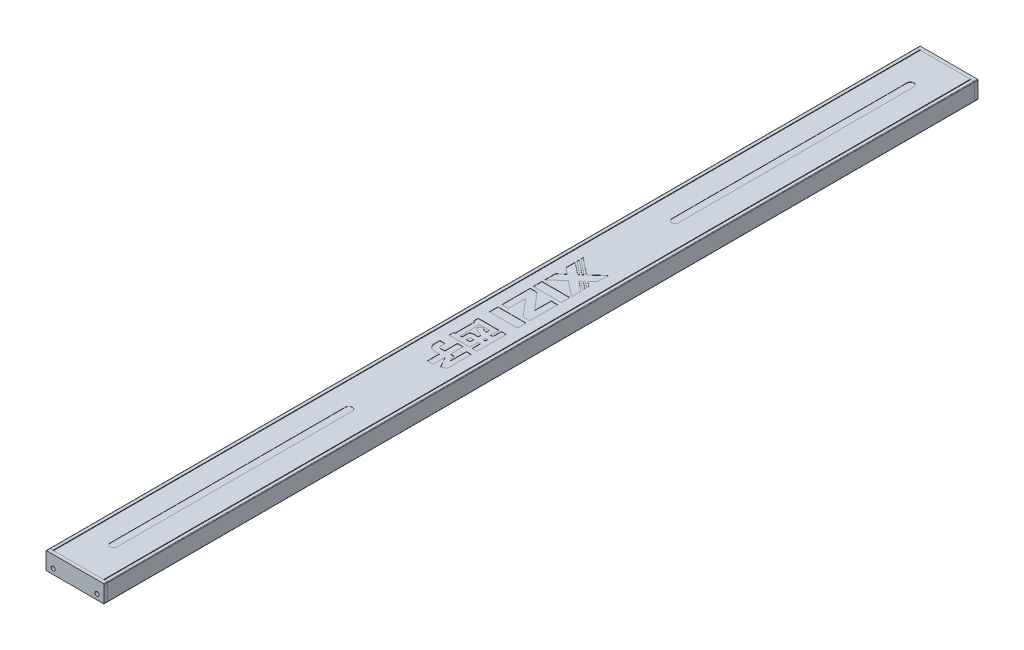
from build123d import *

# Parameters (mm, degrees)
EXTRUDE_1_DEPTH     = 372
SKETCH_3_W          = 43
SKETCH_3_H          = 744
EXTRUDE_4_DEPTH     = 6
SKETCH_7_W          = 50
SKETCH_7_H          = 15
SKETCH_7_R          = 1.75
EXTRUDE_3_DEPTH     = 3
FILLET_2_R          = 0.5
FILLET_3_R          = 0.5
SKETCH_13_W         = 24
SKETCH_13_H         = 7.373249396
SKETCH_13_H_2       = 7.373336991
SKETCH_13_W_2       = 1.89342737
SKETCH_13_H_3       = 1.872448876
CUT_EXTRUDE_1_DEPTH = 0.2


with BuildPart() as part:
    # 草图1 → 凸台-拉伸1 (new, symmetric)
    with BuildSketch(Plane.XY):
        with BuildLine():
            Line((22, 15), (24.5, 15))
            ThreePointArc((24.5, 15), (24.853553391, 14.853553391), (25, 14.5))
            Line((25, 14.5), (25, 0.5))
            ThreePointArc((25, 0.5), (24.853553391, 0.146446609), (24.5, 0))
            Line((24.5, 0), (20.866025404, 0))
            ThreePointArc((20.866025404, 0), (20, 0.5), (19.133974596, 0))
            Line((19.133974596, 0), (17.866025404, 0))
            ThreePointArc((17.866025404, 0), (17, 0.5), (16.133974596, 0))
            Line((16.133974596, 0), (14.866025404, 0))
            ThreePointArc((14.866025404, 0), (14, 0.5), (13.133974596, 0))
            Line((13.133974596, 0), (11.866025404, 0))
            ThreePointArc((11.866025404, 0), (11, 0.5), (10.133974596, 0))
            Line((10.133974596, 0), (-10.133974596, 0))
            ThreePointArc((-10.133974596, 0), (-11, 0.5), (-11.866025404, 0))
            Line((-11.866025404, 0), (-13.133974596, 0))
            ThreePointArc((-13.133974596, 0), (-14, 0.5), (-14.866025404, 0))
            Line((-14.866025404, 0), (-16.133974596, 0))
            ThreePointArc((-16.133974596, 0), (-17, 0.5), (-17.866025404, 0))
            Line((-17.866025404, 0), (-19.133974596, 0))
            ThreePointArc((-19.133974596, 0), (-20, 0.5), (-20.866025404, 0))
            Line((-20.866025404, 0), (-24.5, 0))
            ThreePointArc((-24.5, 0), (-24.853553391, 0.146446609), (-25, 0.5))
            Line((-25, 0.5), (-25, 14.5))
            ThreePointArc((-25, 14.5), (-24.853553391, 14.853553391), (-24.5, 15))
            Line((-24.5, 15), (-22, 15))
            Line((-22, 15), (-22, 9))
            Line((-22, 9), (-13, 9))
            Line((-13, 9), (-13, 8))
            Line((-13, 8), (-14.8, 8))
            ThreePointArc((-14.8, 8), (-14.941421356, 7.941421356), (-15, 7.8))
            Line((-15, 7.8), (-15, 2.7))
            ThreePointArc((-15, 2.7), (-14.941421356, 2.558578644), (-14.8, 2.5))
            Line((-14.8, 2.5), (14.8, 2.5))
            ThreePointArc((14.8, 2.5), (14.941421356, 2.558578644), (15, 2.7))
            Line((15, 2.7), (15, 7.8))
            ThreePointArc((15, 7.8), (14.941421356, 7.941421356), (14.8, 8))
            Line((14.8, 8), (13, 8))
            Line((13, 8), (13, 9))
            Line((13, 9), (22, 9))
            Line((22, 9), (22, 15))
        make_face()
        with BuildLine():
            Line((-21.011700936, 7), (-23, 7))
            Line((-23, 7), (-23, 2))
            Line((-23, 2), (-21.011700936, 2))
            Line((-21.011700936, 2), (-21.011700936, 2.838299064))
            ThreePointArc((-21.011700936, 2.838299064), (-20.672176824, 3.346432807), (-20.072792206, 3.227207794))
            ThreePointArc((-20.072792206, 3.227207794), (-17, 4.5), (-20.072792206, 5.772792206))
            ThreePointArc((-20.072792206, 5.772792206), (-20.672176824, 5.653567193), (-21.011700936, 6.161700936))
            Line((-21.011700936, 6.161700936), (-21.011700936, 7))
        make_face(mode=Mode.SUBTRACT)
        with BuildLine():
            Line((21.011700936, 2.838299064), (21.011700936, 2))
            Line((21.011700936, 2), (23, 2))
            Line((23, 2), (23, 7))
            Line((23, 7), (21.011700936, 7))
            Line((21.011700936, 7), (21.011700936, 6.161700936))
            ThreePointArc((21.011700936, 6.161700936), (20.672176824, 5.653567193), (20.072792206, 5.772792206))
            ThreePointArc((20.072792206, 5.772792206), (17, 4.5), (20.072792206, 3.227207794))
            ThreePointArc((20.072792206, 3.227207794), (20.672176824, 3.346432807), (21.011700936, 2.838299064))
        make_face(mode=Mode.SUBTRACT)
    extrude(amount=EXTRUDE_1_DEPTH, both=True)

    # 草图3 → 凸台-拉伸4 (add)
    with BuildSketch(Plane(origin=(0, 9, 363), x_dir=(1, 0, 0), z_dir=(0, -1, 0))):
        with Locations((0, -363)):
            Rectangle(SKETCH_3_W, SKETCH_3_H)
    extrude(amount=-EXTRUDE_4_DEPTH)

    # 草图13 → 切除-拉伸1 (cut)
    # profile 1 of 8: a face of its own
    with BuildSketch(Plane(origin=(0, 15, 0), x_dir=(1, 0, 0), z_dir=(0, 1, 0))):
        with BuildLine():
            Line((2.974241772, -342), (2.974241772, -140))
            ThreePointArc((2.974241772, -140), (0, -137.025758228), (-2.974241772, -140))
            Line((-2.974241772, -140), (-2.974241772, -342))
            ThreePointArc((-2.974241772, -342), (0, -344.974241772), (2.974241772, -342))
        make_face()
    # profile 2 of 8: a face of its own
    with BuildSketch(Plane(origin=(0, 15, 0), x_dir=(1, 0, 0), z_dir=(0, 1, 0))):
        with BuildLine():
            Line((-2.974241772, 140), (-2.974241772, 342))
            ThreePointArc((-2.974241772, 342), (0, 344.974241772), (2.974241772, 342))
            Line((2.974241772, 342), (2.974241772, 140))
            ThreePointArc((2.974241772, 140), (0, 137.025758228), (-2.974241772, 140))
        make_face()
    # profile 3 of 8: a face of its own
    with BuildSketch(Plane(origin=(0, 15, 0), x_dir=(1, 0, 0), z_dir=(0, 1, 0))):
        Polygon((4.456261904, 54.720624259), (12, 48.692451578), (12, 50.577345914), (5.57614696, 55.708810517), (6.471044745, 56.504083804), (12, 52.088692179), (12, 53.973586515), (7.592433512, 57.493890566), (12, 61.392166226), (12, 70.550396944), (2.156182764, 61.840932727), (-12, 73.159495911), (-12, 71.271287619), (1.035290368, 60.84821705), (0.138772079, 60.056257767), (-12, 69.759430422), (-12, 67.87021479), (-0.977988762, 59.063034807), (-1.931998445, 58.223526141), (-12, 66.268295531), (-12, 58.243322568), (-6.697535727, 54.009485788), (-12, 49.317425953), (-12, 40.158308155), (-1.256657054, 49.660330439), (12, 39.065460697), (12, 47.089013968), (3.504266901, 53.877684796), align=None)
    # profile 4 of 8: a face of its own
    with BuildSketch(Plane(origin=(0, 15, 0), x_dir=(1, 0, 0), z_dir=(0, 1, 0))):
        Polygon((-7.091113811, 27.560714457), (-12, 27.560714457), (-12, 3.255607132), (-6.354237064, 3.255607132), (-6.354237064, 18.06583115), (5.641186107, 3.943620573), (5.720368151, 3.880373274), (5.799825971, 3.817856759), (5.879835345, 3.756801814), (5.960672049, 3.697939223), (6.042611859, 3.641999771), (6.125930553, 3.589714243), (6.210903907, 3.541813424), (6.297807698, 3.499028098), (6.386917702, 3.46208905), (6.478457135, 3.431587784), (6.572269113, 3.40710857), (6.668029606, 3.387792753), (6.765413861, 3.372779768), (6.864097125, 3.361209049), (6.963754646, 3.352220028), (7.064061673, 3.34495214), (7.164693452, 3.338544819), (11.196478202, 3.338544819), (11.223669799, 3.339917348), (11.250846223, 3.341381873), (11.2779923, 3.343030389), (11.305092856, 3.344954893), (11.332132718, 3.347247381), (11.359096712, 3.349999849), (11.385969665, 3.353304291), (11.412736404, 3.357252705), (11.439381754, 3.361937086), (11.465890473, 3.367449179), (11.492239241, 3.373851359), (11.518389194, 3.381149507), (11.544299709, 3.38934309), (11.56993016, 3.398431574), (11.59523992, 3.408414428), (11.620188365, 3.419291116), (11.644734869, 3.431061107), (11.668838572, 3.443723843), (11.692451175, 3.45727802), (11.715515564, 3.471721447), (11.73797411, 3.487051882), (11.759769188, 3.503267084), (11.780843172, 3.520364811), (11.801138435, 3.53834282), (11.820604897, 3.55719357), (11.839230455, 3.576882837), (11.857014933, 3.597368024), (11.873958156, 3.618606529), (11.890059952, 3.640555751), (11.905319631, 3.663173089), (11.919704014, 3.686416074), (11.933128711, 3.710242436), (11.945504821, 3.734609924), (11.956743447, 3.759476287), (11.966755688, 3.784799273), (11.975452645, 3.810536632), (11.98274542, 3.836646112), (11.988560256, 3.863084145), (11.993091003, 3.889783875), (11.996760751, 3.916658501), (12, 3.943620573), (12, 27.157997315), (6.420283552, 27.157997315), (6.420283552, 12.936176839), (-5.19836514, 26.549797346), (-5.264670578, 26.619047642), (-5.331282366, 26.687996834), (-5.398506856, 26.756343814), (-5.466650399, 26.823787478), (-5.536019347, 26.89002672), (-5.606920049, 26.954760435), (-5.679658858, 27.017687517), (-5.754522156, 27.078497538), (-5.831584371, 27.136781093), (-5.910792177, 27.192069125), (-5.99209049, 27.243891756), (-6.075424227, 27.291779106), (-6.160738304, 27.335261297), (-6.247977287, 27.373870896), (-6.337039668, 27.407461402), (-6.427732444, 27.436523635), (-6.519851817, 27.461623627), (-6.613193987, 27.483327413), (-6.707555155, 27.502201028), (-6.80273152, 27.518810505), (-6.898519285, 27.53372188), (-6.994714648, 27.547501186), align=None)
    # profile 5 of 8: a face of its own
    with BuildSketch(Plane(origin=(0, 15, 0), x_dir=(1, 0, 0), z_dir=(0, 1, 0))):
        with Locations((0, 34.027642246)):
            Rectangle(SKETCH_13_W, SKETCH_13_H)
    # profile 6 of 8: a face of its own
    with BuildSketch(Plane(origin=(0, 15, 0), x_dir=(1, 0, 0), z_dir=(0, 1, 0))):
        with Locations((0, -3.686668496)):
            Rectangle(SKETCH_13_W, SKETCH_13_H_2)
    # profile 7 of 8: a face of its own
    with BuildSketch(Plane(origin=(0, 15, 0), x_dir=(1, 0, 0), z_dir=(0, 1, 0))):
        Polygon((5.924614588, -24.169022516), (7.818041958, -24.169022516), (7.818041958, -16.97256707), (11.982569257, -16.97256707), (11.982569257, -41.970375504), (7.818041958, -41.970375504), (7.818041958, -34.790088407), (5.924614588, -34.790088407), (5.924614588, -41.995012989), (1.738743725, -41.995012989), (-12, -41.995012989), (-12, -37.858225237), (-10.849979823, -37.858225237), (-10.849979823, -21.132452464), (-12, -21.132452464), (-12, -16.973336991), (1.738743725, -16.973336991), (5.924614588, -16.973336991), align=None)
        with Locations((6.871328273, -29.660871954)):
            Rectangle(SKETCH_13_W_2, SKETCH_13_H_3, mode=Mode.SUBTRACT)
        with BuildLine():
            Line((-0.261625913, -34.789318486), (1.738743725, -34.789318486))
            Line((1.738743725, -34.789318486), (1.738743725, -37.858225237))
            Line((1.738743725, -37.858225237), (-1.334729515, -37.858225237))
            Line((-1.334729515, -37.858225237), (-1.334729515, -35.862422087))
            ThreePointArc((-1.334729515, -35.862422087), (-1.020424747, -35.103623253), (-0.261625913, -34.789318486))
        make_face(mode=Mode.SUBTRACT)
        with BuildLine():
            Line((1.738743725, -23.831027016), (1.738743725, -21.132452464))
            Line((1.738743725, -21.132452464), (-6.662661938, -21.132452464))
            Line((-6.662661938, -21.132452464), (-6.662661938, -37.858225237))
            Line((-6.662661938, -37.858225237), (-5.130628138, -37.858225237))
            Line((-5.130628138, -37.858225237), (-5.130628138, -33.320661231))
            ThreePointArc((-5.130628138, -33.320661231), (-4.344866218, -31.423664147), (-2.447869134, -30.637902227))
            Line((-2.447869134, -30.637902227), (1.738743725, -30.637902227))
            Line((1.738743725, -30.637902227), (1.738743725, -28.354315317))
            ThreePointArc((1.738743725, -28.354315317), (-2.434085355, -27.022218982), (-5.738377083, -24.146694795))
            Line((-5.738377083, -24.146694795), (-3.061749435, -21.452739772))
            ThreePointArc((-3.061749435, -21.452739772), (-0.879727799, -23.082363135), (1.738743725, -23.831027016))
        make_face(mode=Mode.SUBTRACT)
    # profile 8 of 8: a face of its own
    with BuildSketch(Plane(origin=(0, 15, 0), x_dir=(1, 0, 0), z_dir=(0, 1, 0))):
        with BuildLine():
            Line((7.710238871, -46.892483096), (11.959778671, -46.892483096))
            Line((11.959778671, -46.892483096), (11.959778671, -67.497119948))
            Line((11.959778671, -67.497119948), (8.085740898, -69.371108667))
            Line((8.085740898, -69.371108667), (2.827265497, -60.221362596))
            Line((2.827265497, -60.221362596), (2.827265497, -70.452078331))
            Line((2.827265497, -70.452078331), (-2.177257666, -70.452078331))
            Line((-2.177257666, -70.452078331), (-2.177257666, -60.152069669))
            Line((-2.177257666, -60.152069669), (-6.524146619, -60.152069669))
            ThreePointArc((-6.524146619, -60.152069669), (-10.318140786, -58.580545829), (-11.889664626, -54.786551662))
            Line((-11.889664626, -54.786551662), (-11.889664626, -49.959850005))
            Line((-11.889664626, -49.959850005), (-7.383278545, -49.959850005))
            Line((-7.383278545, -49.959850005), (-7.383278545, -54.264304224))
            ThreePointArc((-7.383278545, -54.264304224), (-6.990397585, -55.212802766), (-6.041899043, -55.605683726))
            Line((-6.041899043, -55.605683726), (-2.177257666, -55.605683726))
            Line((-2.177257666, -55.605683726), (-2.177257666, -44.662790684))
            Line((-2.177257666, -44.662790684), (2.827265497, -44.662790684))
            Line((2.827265497, -44.662790684), (2.827265497, -55.605683726))
            Line((2.827265497, -55.605683726), (6.253450178, -55.605683726))
            Line((6.253450178, -55.605683726), (6.253450178, -57.95086435))
            Line((6.253450178, -57.95086435), (7.710238871, -60.786484913))
            Line((7.710238871, -60.786484913), (7.710238871, -46.892483096))
        make_face()
    extrude(amount=-CUT_EXTRUDE_1_DEPTH, mode=Mode.SUBTRACT)


with BuildPart() as body_2:
    # 草图7 → 凸台-拉伸3 (new body)
    with BuildSketch(Plane.XY.offset(372)):
        with Locations((0, 7.5)):
            Rectangle(SKETCH_7_W, SKETCH_7_H)
        with Locations((-18.8, 4.5)):
            Circle(SKETCH_7_R, mode=Mode.SUBTRACT)
        with Locations((18.8, 4.5)):
            Circle(SKETCH_7_R, mode=Mode.SUBTRACT)
    extrude(amount=EXTRUDE_3_DEPTH)


with BuildPart() as body_3:
    # 镜向1: mirrored copy
    add(body_2.part.mirror(Plane.XY))

    # 圆角3
    fillet_3_edges = [body_3.edges().sort_by_distance(p)[0] for p in [
        (25, 0, -373.5),
        (-25, 0, -373.5),
        (-25, 15, -373.5),
        (25, 15, -373.5),
    ]]
    fillet(fillet_3_edges, radius=FILLET_3_R)


with BuildPart() as body_2_1:
    add(body_2.part)

    # 圆角2
    fillet_2_edges = [body_2_1.edges().sort_by_distance(p)[0] for p in [
        (25, 0, 373.5),
        (-25, 0, 373.5),
        (-25, 15, 373.5),
        (25, 15, 373.5),
    ]]
    fillet(fillet_2_edges, radius=FILLET_2_R)


solid = Compound([part.part, body_3.part, body_2_1.part])
